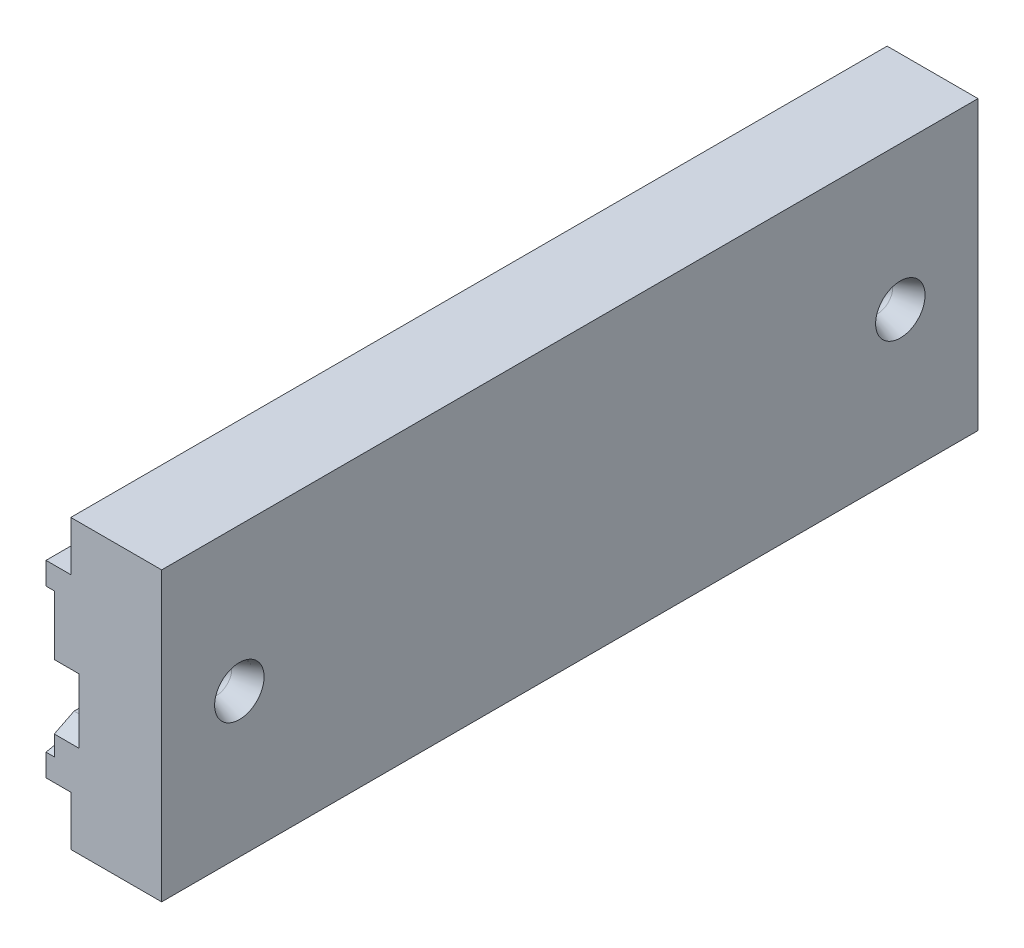
from build123d import *
from OCP.BRepFilletAPI import BRepFilletAPI_MakeChamfer

# Parameters (mm, degrees)
SKETCH1_W           = 49.4
SKETCH1_H           = 17.4
BOSS_EXTRUDE1_DEPTH = 7
SKETCH2_W           = 49.4
SKETCH2_H           = 8.1
CUT_EXTRUDE1_DEPTH  = 0.2
SKETCH3_W           = 49.4
SKETCH3_H           = 3.3
CUT_EXTRUDE2_DEPTH  = 1.7
SKETCH5_W           = 49.4
SKETCH5_H           = 3
CUT_EXTRUDE3_DEPTH  = 1.5
CHAMFER1_SIZE       = 1.5
CHAMFER1_SIZE2      = 0.3
CHAMFER2_SIZE       = 0.3
CHAMFER2_SIZE2      = 1.5


with BuildPart() as part:
    # Sketch1 → Boss-Extrude1 (new body)
    with BuildSketch(Plane(origin=(0, 0, 0), x_dir=(0, 0, -1), z_dir=(1, 0, 0))):
        Rectangle(SKETCH1_W, SKETCH1_H)
    extrude(amount=BOSS_EXTRUDE1_DEPTH)

    # Sketch2 → Cut-Extrude1 (cut)
    with BuildSketch(Plane.ZY):
        Rectangle(SKETCH2_W, SKETCH2_H)
    extrude(amount=-CUT_EXTRUDE1_DEPTH, mode=Mode.SUBTRACT)

    # Sketch3 → Cut-Extrude2 (cut)
    with BuildSketch(Plane.ZY):
        with Locations((0, -1.2)):
            Rectangle(SKETCH3_W, SKETCH3_H)
    extrude(amount=-CUT_EXTRUDE2_DEPTH, mode=Mode.SUBTRACT)

    # Sketch4 → Cut-Revolve1 (revolve, cut)
    with BuildSketch(Plane(origin=(0, 0, 0), x_dir=(1, 0, 0), z_dir=(0, 1, 0))):
        with BuildLine():
            Line((5.617316568, 20.923879533), (7, 21.496605763))
            Line((7, 21.496605763), (7, 20))
            Line((7, 20), (5, 20))
            ThreePointArc((5, 20), (5.168530388, 20.555570233), (5.617316568, 20.923879533))
        make_face()
    cut_revolve1 = revolve(axis=Axis((9.957130438, 0, -20), (1, 0, 0)), mode=Mode.SUBTRACT)

    # Mirror1: Cut-Revolve1 across plane
    add(cut_revolve1.mirror(Plane.XY), mode=Mode.SUBTRACT)

    # Sketch5 → Cut-Extrude3 (cut)
    with BuildSketch(Plane.ZY):
        with Locations((0, 7.2)):
            Rectangle(SKETCH5_W, SKETCH5_H)
        with Locations((0, -7.2)):
            Rectangle(SKETCH5_W, SKETCH5_H)
    extrude(amount=-CUT_EXTRUDE3_DEPTH, mode=Mode.SUBTRACT)

    # Chamfer1: one chamfer whose edges measure the first distance from different faces: ONE call of the kernel's chamfer builder (chamfer() names one face for all edges)
    chamfer1_edges_1 = [part.edges().sort_by_distance(p)[0] for p in [
        (0.2, -3.45, 24.7),
    ]]
    chamfer1_side_1 = [part.faces().sort_by_distance(p)[0] for p in [
        (0.2, -3.45, 0),
    ]]
    chamfer1_edges_2 = [part.edges().sort_by_distance(p)[0] for p in [
        (0.1, -4.05, 24.7),
    ]]
    chamfer1_side_2 = [part.faces().sort_by_distance(p)[0] for p in [
        (0.1, -4.05, 0),
    ]]
    chamfer1_edges_3 = [part.edges().sort_by_distance(p)[0] for p in [
        (0.95, -2.85, 24.7),
    ]]
    chamfer1_side_3 = [part.faces().sort_by_distance(p)[0] for p in [
        (0.95, -2.85, 0),
    ]]
    chamfer1 = BRepFilletAPI_MakeChamfer(part.part.solid().wrapped)
    for e in chamfer1_edges_1:
        chamfer1.Add(CHAMFER1_SIZE, CHAMFER1_SIZE2, e.wrapped, chamfer1_side_1[0].wrapped)  # the first distance lies on this face
    for e in chamfer1_edges_2:
        chamfer1.Add(CHAMFER1_SIZE, CHAMFER1_SIZE2, e.wrapped, chamfer1_side_2[0].wrapped)  # the first distance lies on this face
    for e in chamfer1_edges_3:
        chamfer1.Add(CHAMFER1_SIZE, CHAMFER1_SIZE2, e.wrapped, chamfer1_side_3[0].wrapped)  # the first distance lies on this face
    add(Compound.cast(chamfer1.Shape()), mode=Mode.REPLACE)

    # Chamfer2
    chamfer2_edges = [part.edges().sort_by_distance(p)[0] for p in [
        (1.7, -1.35, 24.7),
        (0.1, 4.05, 24.7),
        (0.2, 2.25, 24.7),
        (0.95, 0.45, 24.7),
    ]]
    chamfer2_side = [part.faces().sort_by_distance(p)[0] for p in [
        (3.930580866, 0.084396355, 24.7),
    ]]
    chamfer(chamfer2_edges, length=CHAMFER2_SIZE, length2=CHAMFER2_SIZE2, reference=chamfer2_side[0])


solid = part.part
